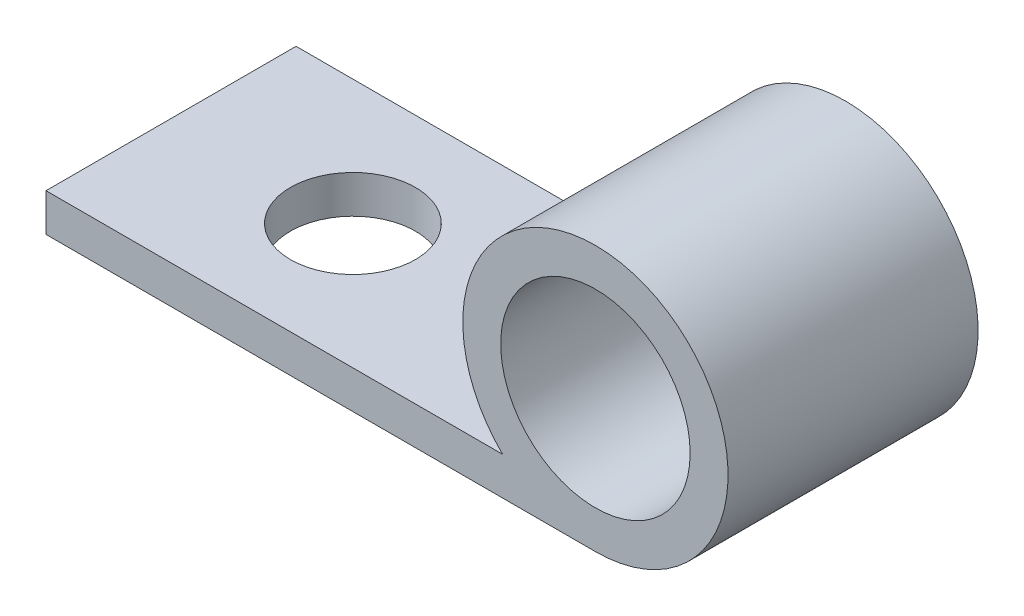
SolidWorks part; units mm, degrees
ref_plane "前视基准面" through (0, 0, 0) normal (0, 0, 1) x (1, 0, 0)
ref_plane "上视基准面" through (0, 0, 0) normal (0, 1, 0) x (1, 0, 0)
ref_plane "右视基准面" through (0, 0, 0) normal (1, 0, 0) x (0, 0, -1)
sketch "草图1" plane through (0, 0, 0) normal (0, 0, 1) x (1, 0, 0)
  line L0 (0, 0) -> (14.5, 0)
  line L1 (0, 1) -> (14.5, 1)
  line L2 (0, 1) -> (0, 0)
  circle A1 centre (14.5, 3.5) radius 3.5
  circle A2 centre (14.5, 3.5) radius 2.5
  dimension "D1" = 1
  dimension "D3" = 14.5
  dimension "D4" = 7
  dimension "D2" = 1
extrude "凸台-拉伸1" add sketch "草图1" along normal mid plane 6.6
sketch "草图2" plane through (0, 1, 0) normal (0, 1, 0) x (1, 0, 0)
  line L0 (0, 0) -> (4.8, 0) construction
  circle A0 centre (4.8, 0) radius 1.65
  dimension "D1" = 3.3
  dimension "D2" = 4.8
extrude "切除-拉伸1" cut sketch "草图2" against normal blind 6.6
